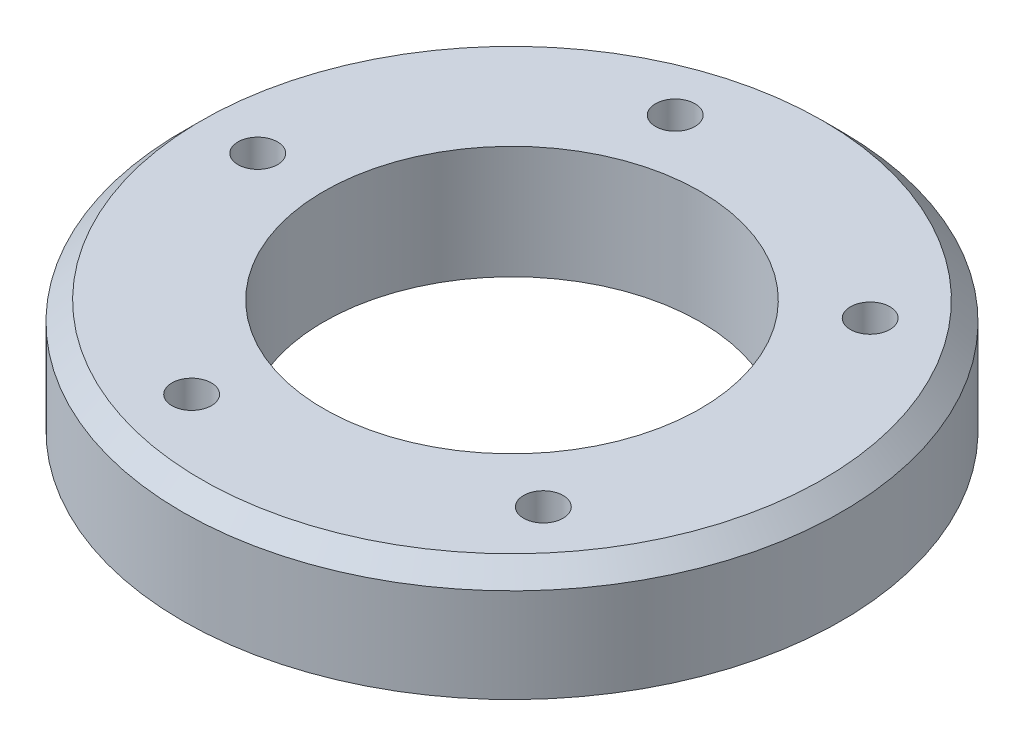
from build123d import *

# Parameters (mm, degrees)
SKETCH2_R             = 1.75
CUT_EXTRUDE1_DEPTH    = 10
M5_TAPPED_HOLE1_D     = 4.2
M5_TAPPED_HOLE1_DEPTH = 10
M5_TAPPED_HOLE1_TIP   = 1.2618073


with BuildPart() as part:
    # Sketch1 → Revolve1 (revolve)
    with BuildSketch(Plane(origin=(0, 0, 0), x_dir=(0, 0, -1), z_dir=(1, 0, 0))):
        Polygon((35, 10), (33, 12), (20, 12), (20, 0), (35, 0), align=None)
    revolve(axis=Axis((0, 0, 0), (0, 1, 0)))

    # Sketch2 → Cut-Extrude1 (cut)
    with BuildSketch(Plane(origin=(0, 12, 0), x_dir=(1, 0, 0), z_dir=(0, 1, 0))):
        with Locations(Location((-27, 0, 0), (0, 0, 270))):
            Circle(SKETCH2_R)
        with Locations(Location((-8.343458848, 25.67852594, 0), (0, 0, 270))):
            Circle(SKETCH2_R)
        with Locations(Location((-8.343458848, -25.67852594, 0), (0, 0, 90))):
            Circle(SKETCH2_R)
        with Locations(Location((20.683199964, 17.355265462, 0), (0, 0, 270))):
            Circle(SKETCH2_R)
        with Locations(Location((20.683199964, -17.355265462, 0), (0, 0, 90))):
            Circle(SKETCH2_R)
    extrude(amount=-CUT_EXTRUDE1_DEPTH, mode=Mode.SUBTRACT)

    # M5 Tapped Hole1
    with Locations(Plane(origin=(0, 12, 0), x_dir=(1, 0, 0), z_dir=(0, 1, 0))):
        with Locations((-27, 0), (-8.343458848, 25.67852594), (20.683199964, 17.355265462), (20.683199964, -17.355265462), (-8.343458848, -25.67852594)):
            Hole(M5_TAPPED_HOLE1_D / 2, depth=M5_TAPPED_HOLE1_DEPTH)
            with Locations((0, 0, -(M5_TAPPED_HOLE1_DEPTH + M5_TAPPED_HOLE1_TIP / 2))):  # 118° drill point
                Cone(0, M5_TAPPED_HOLE1_D / 2, M5_TAPPED_HOLE1_TIP, mode=Mode.SUBTRACT)


solid = part.part
